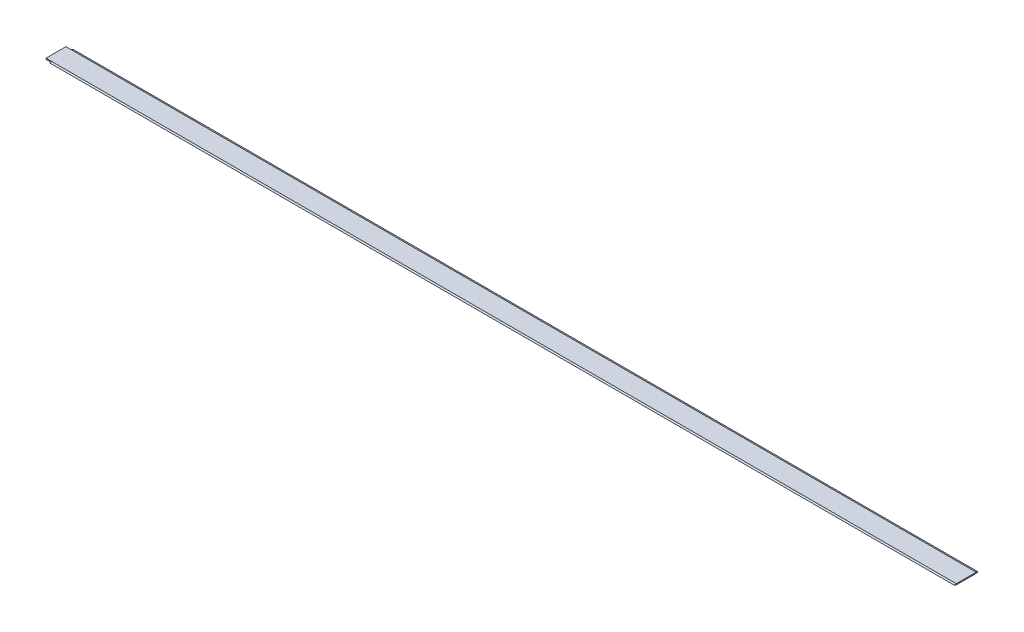
from build123d import *

# Parameters (mm, degrees)
SKETCH1_W               = 500
SKETCH1_H               = 13
BOSS_EXTRUDE1_DEPTH     = 0.3
CUT_EXTRUDE1_DEPTH      = 251.084665663
CUT_EXTRUDE1_DEPTH_BACK = 251.084665663
SKETCH3_W               = 11
SKETCH3_H               = 0.6
BOSS_EXTRUDE2_DEPTH     = 3


with BuildPart() as part:
    # Sketch1 → Boss-Extrude1 (new, symmetric)
    with BuildSketch(Plane(origin=(0, 0, 0), x_dir=(1, 0, 0), z_dir=(0, 1, 0))):
        Rectangle(SKETCH1_W, SKETCH1_H)
    extrude(amount=BOSS_EXTRUDE1_DEPTH, both=True)

    # Sketch2 → Cut-Extrude1 (cut, two sides: drawn at the far end of the back side and taken through both)
    with BuildSketch(Plane(origin=(0, 0, 0), x_dir=(0, 0, -1), z_dir=(1, 0, 0)).offset(-CUT_EXTRUDE1_DEPTH_BACK)):
        Polygon((5.5, 0.3), (6.5, 0), (5.5, -0.3), (7, -0.3), (7, 0.3), align=None)
        Polygon((-7, 0.3), (-5.5, 0.3), (-6.5, 0), (-5.5, -0.3), (-7, -0.3), align=None)
    extrude(amount=CUT_EXTRUDE1_DEPTH + CUT_EXTRUDE1_DEPTH_BACK, mode=Mode.SUBTRACT)

    # Sketch3 → Boss-Extrude2 (add)
    with BuildSketch(Plane.ZY.offset(250)):
        Rectangle(SKETCH3_W, SKETCH3_H)
    extrude(amount=BOSS_EXTRUDE2_DEPTH)


solid = part.part
